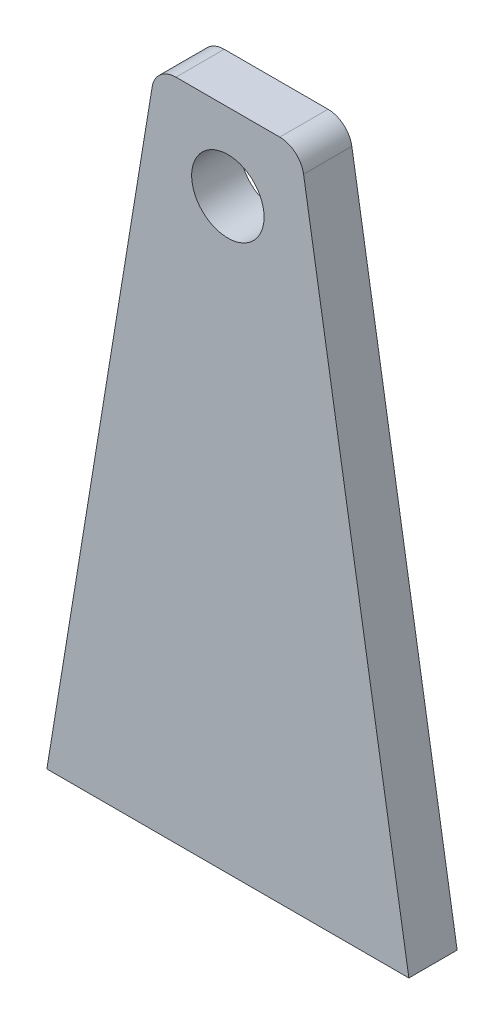
SolidWorks part; units mm, degrees
material "Q235B"
ref_plane "Front Plane" through (0, 0, 0) normal (0, 0, 1) x (1, 0, 0)
ref_plane "Top Plane" through (0, 0, 0) normal (0, 1, 0) x (1, 0, 0)
ref_plane "Right Plane" through (0, 0, 0) normal (1, 0, 0) x (0, 0, -1)
sketch "Sketch1" plane through (0, 0, 0) normal (0, 0, 1) x (1, 0, 0)
  line L1 (0, 0) -> (300, 0)
  line L2 (0, 0) -> (87.2558, 533.2298)
  line L3 (106.9933, 550) -> (193.0067, 550)
  line L4 (300, 0) -> (212.7442, 533.2298)
  arc A0 (193.0067, 550) -> (212.7442, 533.2298) centre (193.0067, 530) cw
  arc A1 (87.2558, 533.2298) -> (106.9933, 550) centre (106.9933, 530) cw
  circle A2 centre (150, 486) radius 30
  point P7 (210, 550)
  point P10 (90, 550)
  dimension "D3" = 20
  dimension "D4" = 60
  dimension "D5" = 486
  dimension "D6" = 60
  dimension "D8" = 150
  dimension "D1" = 550
  dimension "D2" = 120
  dimension "D7" = 300
extrude "Boss-Extrude1" add sketch "Sketch1" along normal blind 40
